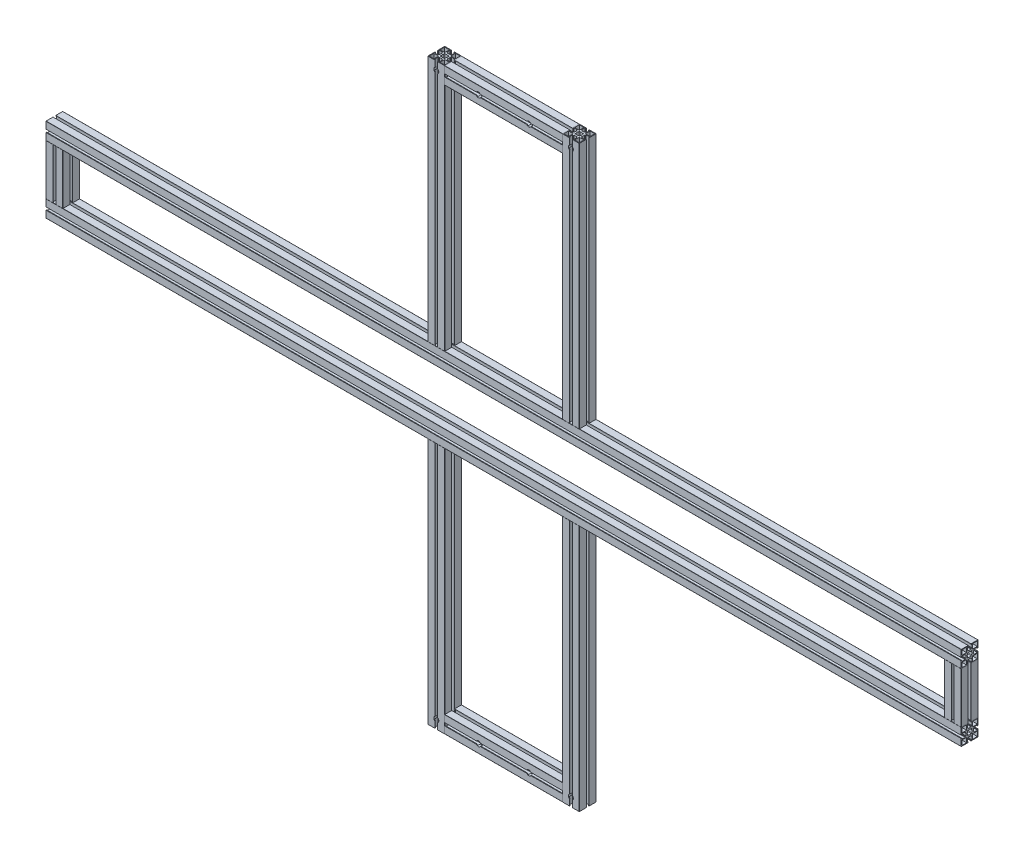
SolidWorks part; units mm, degrees
ref_plane "前视" through (0, 0, 0) normal (0, 0, 1) x (1, 0, 0)
ref_plane "上视" through (0, 0, 0) normal (0, 1, 0) x (1, 0, 0)
ref_plane "右视" through (0, 0, 0) normal (1, 0, 0) x (0, 0, -1)
sketch3d "3D草图1"
  line L0 (0, 0, 0) -> (2670, 0, 0)
  line L1 (2670, 0, 0) -> (2670, -200, 0)
  line L2 (2670, -200, 0) -> (0, -200, 0)
  line L3 (0, -200, 0) -> (0, 0, 0)
  line L4 (1135, 0, 0) -> (1135, 735, 0)
  line L5 (1135, 735, 0) -> (1535, 735, 0)
  line L6 (1535, 735, 0) -> (1535, 0, 0)
  line L7 (1135, -200, 0) -> (1135, -935, 0)
  line L8 (1135, -935, 0) -> (1535, -935, 0)
  line L9 (1535, -935, 0) -> (1535, -200, 0)
  line L10 (1335, 735, 0) -> (1335, 0, 0) construction
  dimension "D1" = 2670
  dimension "D2" = 200
  dimension "D3" = 400
  dimension "D4" = 1670
other "结构构件1"
ref_plane "基准面1" through (2670, -200, 0) normal (-1, 0, 0) x (0, 0, 1)
sketch "Sketch13" plane through (2670, -200, 0) normal (-1, 0, 0) x (0, 0, 1)
  line L0 (0, 0) -> (0, 16.3773) construction
  line L1 (0, 0) -> (-5.6569, 5.6569) construction
  line L2 (-24.5, 25) -> (-4.25, 25)
  line L3 (-25, 24.5) -> (-25, 4.25)
  line L4 (-24.5, -25) -> (-4.25, -25)
  line L5 (25, 24.5) -> (25, 4.25)
  line L6 (-4.879, 6.4347) -> (-4.1104, 5.6661)
  line L7 (-6.4347, 4.879) -> (-5.6661, 4.1104)
  line L8 (6.4347, 4.879) -> (5.6661, 4.1104)
  line L9 (0, 0) -> (20.7093, 0) construction
  line L10 (4.879, 6.4347) -> (4.1104, 5.6661)
  line L11 (4.879, -6.4347) -> (4.1104, -5.6661)
  line L12 (6.4347, -4.879) -> (5.6661, -4.1104)
  line L13 (-6.4347, -4.879) -> (-5.6661, -4.1104)
  line L14 (-4.879, -6.4347) -> (-4.1104, -5.6661)
  line L15 (-4.25, 25) -> (-4.25, 23.2)
  line L16 (-23, 23) -> (-9, 23)
  line L17 (-23, 23) -> (-23, 9)
  line L18 (-23, 9) -> (-9, 9)
  line L19 (-9, 23) -> (-9, 9)
  line L20 (-6.85, 23.2) -> (-4.25, 23.2)
  line L21 (-6.85, 23.2) -> (-6.85, 13.2)
  line L22 (-6.85, 13.2) -> (-4.25, 13.2)
  line L23 (6.85, 23.2) -> (6.85, 13.2)
  line L24 (4.25, 25) -> (4.25, 23.2)
  line L25 (4.25, 25) -> (24.5, 25)
  line L26 (4.25, 23.2) -> (6.85, 23.2)
  line L27 (9, 23) -> (9, 9)
  line L28 (23, 9) -> (9, 9)
  line L29 (23, 23) -> (23, 9)
  line L30 (23, 23) -> (9, 23)
  line L31 (23.2, 6.85) -> (13.2, 6.85)
  line L32 (23.2, 6.85) -> (23.2, 4.25)
  line L33 (25, 4.25) -> (23.2, 4.25)
  line L34 (13.2, 6.85) -> (13.2, 4.25)
  line L35 (23.2, -6.85) -> (13.2, -6.85)
  line L36 (23.2, -4.25) -> (23.2, -6.85)
  line L37 (25, -4.25) -> (23.2, -4.25)
  line L38 (6.85, -23.2) -> (6.85, -13.2)
  line L39 (6.85, -23.2) -> (4.25, -23.2)
  line L40 (4.25, -25) -> (4.25, -23.2)
  line L41 (6.85, -13.2) -> (4.25, -13.2)
  line L42 (-6.85, -23.2) -> (-6.85, -13.2)
  line L43 (-4.25, -23.2) -> (-6.85, -23.2)
  line L44 (-4.25, -25) -> (-4.25, -23.2)
  line L45 (-23.2, -6.85) -> (-13.2, -6.85)
  line L46 (-23.2, -6.85) -> (-23.2, -4.25)
  line L47 (-25, -4.25) -> (-23.2, -4.25)
  line L48 (-13.2, -6.85) -> (-13.2, -4.25)
  line L49 (-23.2, 6.85) -> (-13.2, 6.85)
  line L50 (-23.2, 4.25) -> (-23.2, 6.85)
  line L51 (-25, 4.25) -> (-23.2, 4.25)
  line L52 (4.25, -25) -> (24.5, -25)
  line L53 (-25, -4.25) -> (-25, -24.5)
  line L54 (25, -4.25) -> (25, -24.5)
  line L55 (23, -23) -> (23, -9)
  line L56 (23, -9) -> (9, -9)
  line L57 (9, -23) -> (9, -9)
  line L58 (23, -23) -> (9, -23)
  line L59 (-9, -23) -> (-9, -9)
  line L60 (-23, -9) -> (-9, -9)
  line L61 (-23, -23) -> (-9, -23)
  line L62 (-23, -23) -> (-23, -9)
  line L63 (-4.25, 13.2) -> (-4.25, 11.4)
  line L64 (-4.25, 11.4) -> (4.25, 11.4)
  line L65 (4.25, 11.4) -> (4.25, 13.2)
  line L66 (4.25, 13.2) -> (6.85, 13.2)
  line L67 (13.2, 4.25) -> (11.4, 4.25)
  line L68 (11.4, 4.25) -> (11.4, -4.25)
  line L69 (11.4, -4.25) -> (13.2, -4.25)
  line L70 (4.25, -13.2) -> (4.25, -11.4)
  line L71 (4.25, -11.4) -> (-4.25, -11.4)
  line L72 (-4.25, -11.4) -> (-4.25, -13.2)
  line L73 (-13.2, -4.25) -> (-11.4, -4.25)
  line L74 (-11.4, -4.25) -> (-11.4, 4.25)
  line L75 (-11.4, 4.25) -> (-13.2, 4.25)
  line L76 (-13.2, 4.25) -> (-13.2, 6.85)
  line L77 (-4.25, -13.2) -> (-6.85, -13.2)
  line L78 (13.2, -4.25) -> (13.2, -6.85)
  arc A0 (-4.1104, 5.6661) -> (4.1104, 5.6661) centre (0, 0) cw
  arc A1 (-4.879, 6.4347) -> (-6.4347, 4.879) centre (-5.6569, 5.6569) ccw
  arc A2 (-4.1104, -5.6661) -> (4.1104, -5.6661) centre (0, 0) ccw
  arc A3 (-5.6661, 4.1104) -> (-5.6661, -4.1104) centre (0, 0) ccw
  arc A4 (6.4347, 4.879) -> (4.879, 6.4347) centre (5.6569, 5.6569) ccw
  arc A5 (4.879, -6.4347) -> (6.4347, -4.879) centre (5.6569, -5.6569) ccw
  arc A6 (-6.4347, -4.879) -> (-4.879, -6.4347) centre (-5.6569, -5.6569) ccw
  arc A7 (5.6661, 4.1104) -> (5.6661, -4.1104) centre (0, 0) cw
  arc A8 (-24.5, 25) -> (-25, 24.5) centre (-24.5, 24.5) ccw
  arc A9 (24.5, 25) -> (25, 24.5) centre (24.5, 24.5) cw
  arc A10 (24.5, -25) -> (25, -24.5) centre (24.5, -24.5) ccw
  arc A11 (-25, -24.5) -> (-24.5, -25) centre (-24.5, -24.5) ccw
  point P88 (-25, 25)
  point P91 (25, 25)
  point P92 (-25, -25)
  point P105 (25, -25)
  point P106 (0, 0)
  dimension "D2" = 7
  dimension "D3" = 45
  dimension "D4" = 1.1
  dimension "D5" = 1.8
  dimension "D6" = 8
  dimension "D7" = 2
  dimension "D8" = 13.7
  dimension "D10" = 10
  dimension "D11" = 14
  dimension "D12" = 50
  dimension "D13" = 8.5
  dimension "D14" = 0.5
  dimension "D9" = 2
other "结构构件2"
ref_plane "基准面2" through (1135, 0, 0) normal (0, 1, 0) x (1, 0, 0)
sketch "Sketch14" plane through (1135, 0, 0) normal (0, 1, 0) x (1, 0, 0)
  line L0 (0, 0) -> (0, 16.3773) construction
  line L1 (0, 0) -> (-5.6569, 5.6569) construction
  line L2 (-24.5, 25) -> (-4.25, 25)
  line L3 (-25, 24.5) -> (-25, 4.25)
  line L4 (-24.5, -25) -> (-4.25, -25)
  line L5 (25, 24.5) -> (25, 4.25)
  line L6 (-4.879, 6.4347) -> (-4.1104, 5.6661)
  line L7 (-6.4347, 4.879) -> (-5.6661, 4.1104)
  line L8 (6.4347, 4.879) -> (5.6661, 4.1104)
  line L9 (0, 0) -> (20.7093, 0) construction
  line L10 (4.879, 6.4347) -> (4.1104, 5.6661)
  line L11 (4.879, -6.4347) -> (4.1104, -5.6661)
  line L12 (6.4347, -4.879) -> (5.6661, -4.1104)
  line L13 (-6.4347, -4.879) -> (-5.6661, -4.1104)
  line L14 (-4.879, -6.4347) -> (-4.1104, -5.6661)
  line L15 (-4.25, 25) -> (-4.25, 23.2)
  line L16 (-23, 23) -> (-9, 23)
  line L17 (-23, 23) -> (-23, 9)
  line L18 (-23, 9) -> (-9, 9)
  line L19 (-9, 23) -> (-9, 9)
  line L20 (-6.85, 23.2) -> (-4.25, 23.2)
  line L21 (-6.85, 23.2) -> (-6.85, 13.2)
  line L22 (-6.85, 13.2) -> (-4.25, 13.2)
  line L23 (6.85, 23.2) -> (6.85, 13.2)
  line L24 (4.25, 25) -> (4.25, 23.2)
  line L25 (4.25, 25) -> (24.5, 25)
  line L26 (4.25, 23.2) -> (6.85, 23.2)
  line L27 (9, 23) -> (9, 9)
  line L28 (23, 9) -> (9, 9)
  line L29 (23, 23) -> (23, 9)
  line L30 (23, 23) -> (9, 23)
  line L31 (23.2, 6.85) -> (13.2, 6.85)
  line L32 (23.2, 6.85) -> (23.2, 4.25)
  line L33 (25, 4.25) -> (23.2, 4.25)
  line L34 (13.2, 6.85) -> (13.2, 4.25)
  line L35 (23.2, -6.85) -> (13.2, -6.85)
  line L36 (23.2, -4.25) -> (23.2, -6.85)
  line L37 (25, -4.25) -> (23.2, -4.25)
  line L38 (6.85, -23.2) -> (6.85, -13.2)
  line L39 (6.85, -23.2) -> (4.25, -23.2)
  line L40 (4.25, -25) -> (4.25, -23.2)
  line L41 (6.85, -13.2) -> (4.25, -13.2)
  line L42 (-6.85, -23.2) -> (-6.85, -13.2)
  line L43 (-4.25, -23.2) -> (-6.85, -23.2)
  line L44 (-4.25, -25) -> (-4.25, -23.2)
  line L45 (-23.2, -6.85) -> (-13.2, -6.85)
  line L46 (-23.2, -6.85) -> (-23.2, -4.25)
  line L47 (-25, -4.25) -> (-23.2, -4.25)
  line L48 (-13.2, -6.85) -> (-13.2, -4.25)
  line L49 (-23.2, 6.85) -> (-13.2, 6.85)
  line L50 (-23.2, 4.25) -> (-23.2, 6.85)
  line L51 (-25, 4.25) -> (-23.2, 4.25)
  line L52 (4.25, -25) -> (24.5, -25)
  line L53 (-25, -4.25) -> (-25, -24.5)
  line L54 (25, -4.25) -> (25, -24.5)
  line L55 (23, -23) -> (23, -9)
  line L56 (23, -9) -> (9, -9)
  line L57 (9, -23) -> (9, -9)
  line L58 (23, -23) -> (9, -23)
  line L59 (-9, -23) -> (-9, -9)
  line L60 (-23, -9) -> (-9, -9)
  line L61 (-23, -23) -> (-9, -23)
  line L62 (-23, -23) -> (-23, -9)
  line L63 (-4.25, 13.2) -> (-4.25, 11.4)
  line L64 (-4.25, 11.4) -> (4.25, 11.4)
  line L65 (4.25, 11.4) -> (4.25, 13.2)
  line L66 (4.25, 13.2) -> (6.85, 13.2)
  line L67 (13.2, 4.25) -> (11.4, 4.25)
  line L68 (11.4, 4.25) -> (11.4, -4.25)
  line L69 (11.4, -4.25) -> (13.2, -4.25)
  line L70 (4.25, -13.2) -> (4.25, -11.4)
  line L71 (4.25, -11.4) -> (-4.25, -11.4)
  line L72 (-4.25, -11.4) -> (-4.25, -13.2)
  line L73 (-13.2, -4.25) -> (-11.4, -4.25)
  line L74 (-11.4, -4.25) -> (-11.4, 4.25)
  line L75 (-11.4, 4.25) -> (-13.2, 4.25)
  line L76 (-13.2, 4.25) -> (-13.2, 6.85)
  line L77 (-4.25, -13.2) -> (-6.85, -13.2)
  line L78 (13.2, -4.25) -> (13.2, -6.85)
  arc A0 (-4.1104, 5.6661) -> (4.1104, 5.6661) centre (0, 0) cw
  arc A1 (-4.879, 6.4347) -> (-6.4347, 4.879) centre (-5.6569, 5.6569) ccw
  arc A2 (-4.1104, -5.6661) -> (4.1104, -5.6661) centre (0, 0) ccw
  arc A3 (-5.6661, 4.1104) -> (-5.6661, -4.1104) centre (0, 0) ccw
  arc A4 (6.4347, 4.879) -> (4.879, 6.4347) centre (5.6569, 5.6569) ccw
  arc A5 (4.879, -6.4347) -> (6.4347, -4.879) centre (5.6569, -5.6569) ccw
  arc A6 (-6.4347, -4.879) -> (-4.879, -6.4347) centre (-5.6569, -5.6569) ccw
  arc A7 (5.6661, 4.1104) -> (5.6661, -4.1104) centre (0, 0) cw
  arc A8 (-24.5, 25) -> (-25, 24.5) centre (-24.5, 24.5) ccw
  arc A9 (24.5, 25) -> (25, 24.5) centre (24.5, 24.5) cw
  arc A10 (24.5, -25) -> (25, -24.5) centre (24.5, -24.5) ccw
  arc A11 (-25, -24.5) -> (-24.5, -25) centre (-24.5, -24.5) ccw
  point P88 (-25, 25)
  point P91 (25, 25)
  point P92 (-25, -25)
  point P105 (25, -25)
  point P106 (0, 0)
  dimension "D2" = 7
  dimension "D3" = 45
  dimension "D4" = 1.1
  dimension "D5" = 1.8
  dimension "D6" = 8
  dimension "D7" = 2
  dimension "D8" = 13.7
  dimension "D10" = 10
  dimension "D11" = 14
  dimension "D12" = 50
  dimension "D13" = 8.5
  dimension "D14" = 0.5
  dimension "D9" = 2
other "剪裁/延伸1"
other "剪裁/延伸2"
other "铝型材 50 X 50L X R0.5(1)"
ref_plane "基准面4" through (1135, 735, 0) normal (1, 0, 0) x (0, 0, -1)
sketch "Sketch1" plane through (1135, 735, 0) normal (1, 0, 0) x (0, 0, -1)
  line L0 (0, 0) -> (0, 16.3773) construction
  line L1 (0, 0) -> (-5.6569, 5.6569) construction
  line L2 (-24.5, 25) -> (-4.25, 25)
  line L3 (-25, 24.5) -> (-25, 4.25)
  line L4 (-24.5, -25) -> (-4.25, -25)
  line L5 (25, 24.5) -> (25, 4.25)
  line L6 (-4.879, 6.4347) -> (-4.1104, 5.6661)
  line L7 (-6.4347, 4.879) -> (-5.6661, 4.1104)
  line L8 (6.4347, 4.879) -> (5.6661, 4.1104)
  line L9 (0, 0) -> (20.7093, 0) construction
  line L10 (4.879, 6.4347) -> (4.1104, 5.6661)
  line L11 (4.879, -6.4347) -> (4.1104, -5.6661)
  line L12 (6.4347, -4.879) -> (5.6661, -4.1104)
  line L13 (-6.4347, -4.879) -> (-5.6661, -4.1104)
  line L14 (-4.879, -6.4347) -> (-4.1104, -5.6661)
  line L15 (-4.25, 25) -> (-4.25, 23.2)
  line L16 (-23, 23) -> (-9, 23)
  line L17 (-23, 23) -> (-23, 9)
  line L18 (-23, 9) -> (-9, 9)
  line L19 (-9, 23) -> (-9, 9)
  line L20 (-6.85, 23.2) -> (-4.25, 23.2)
  line L21 (-6.85, 23.2) -> (-6.85, 13.2)
  line L22 (-6.85, 13.2) -> (-4.25, 13.2)
  line L23 (6.85, 23.2) -> (6.85, 13.2)
  line L24 (4.25, 25) -> (4.25, 23.2)
  line L25 (4.25, 25) -> (24.5, 25)
  line L26 (4.25, 23.2) -> (6.85, 23.2)
  line L27 (9, 23) -> (9, 9)
  line L28 (23, 9) -> (9, 9)
  line L29 (23, 23) -> (23, 9)
  line L30 (23, 23) -> (9, 23)
  line L31 (23.2, 6.85) -> (13.2, 6.85)
  line L32 (23.2, 6.85) -> (23.2, 4.25)
  line L33 (25, 4.25) -> (23.2, 4.25)
  line L34 (13.2, 6.85) -> (13.2, 4.25)
  line L35 (23.2, -6.85) -> (13.2, -6.85)
  line L36 (23.2, -4.25) -> (23.2, -6.85)
  line L37 (25, -4.25) -> (23.2, -4.25)
  line L38 (6.85, -23.2) -> (6.85, -13.2)
  line L39 (6.85, -23.2) -> (4.25, -23.2)
  line L40 (4.25, -25) -> (4.25, -23.2)
  line L41 (6.85, -13.2) -> (4.25, -13.2)
  line L42 (-6.85, -23.2) -> (-6.85, -13.2)
  line L43 (-4.25, -23.2) -> (-6.85, -23.2)
  line L44 (-4.25, -25) -> (-4.25, -23.2)
  line L45 (-23.2, -6.85) -> (-13.2, -6.85)
  line L46 (-23.2, -6.85) -> (-23.2, -4.25)
  line L47 (-25, -4.25) -> (-23.2, -4.25)
  line L48 (-13.2, -6.85) -> (-13.2, -4.25)
  line L49 (-23.2, 6.85) -> (-13.2, 6.85)
  line L50 (-23.2, 4.25) -> (-23.2, 6.85)
  line L51 (-25, 4.25) -> (-23.2, 4.25)
  line L52 (4.25, -25) -> (24.5, -25)
  line L53 (-25, -4.25) -> (-25, -24.5)
  line L54 (25, -4.25) -> (25, -24.5)
  line L55 (23, -23) -> (23, -9)
  line L56 (23, -9) -> (9, -9)
  line L57 (9, -23) -> (9, -9)
  line L58 (23, -23) -> (9, -23)
  line L59 (-9, -23) -> (-9, -9)
  line L60 (-23, -9) -> (-9, -9)
  line L61 (-23, -23) -> (-9, -23)
  line L62 (-23, -23) -> (-23, -9)
  line L63 (-4.25, 13.2) -> (-4.25, 11.4)
  line L64 (-4.25, 11.4) -> (4.25, 11.4)
  line L65 (4.25, 11.4) -> (4.25, 13.2)
  line L66 (4.25, 13.2) -> (6.85, 13.2)
  line L67 (13.2, 4.25) -> (11.4, 4.25)
  line L68 (11.4, 4.25) -> (11.4, -4.25)
  line L69 (11.4, -4.25) -> (13.2, -4.25)
  line L70 (4.25, -13.2) -> (4.25, -11.4)
  line L71 (4.25, -11.4) -> (-4.25, -11.4)
  line L72 (-4.25, -11.4) -> (-4.25, -13.2)
  line L73 (-13.2, -4.25) -> (-11.4, -4.25)
  line L74 (-11.4, -4.25) -> (-11.4, 4.25)
  line L75 (-11.4, 4.25) -> (-13.2, 4.25)
  line L76 (-13.2, 4.25) -> (-13.2, 6.85)
  line L77 (-4.25, -13.2) -> (-6.85, -13.2)
  line L78 (13.2, -4.25) -> (13.2, -6.85)
  arc A0 (-4.1104, 5.6661) -> (4.1104, 5.6661) centre (0, 0) cw
  arc A1 (-4.879, 6.4347) -> (-6.4347, 4.879) centre (-5.6569, 5.6569) ccw
  arc A2 (-4.1104, -5.6661) -> (4.1104, -5.6661) centre (0, 0) ccw
  arc A3 (-5.6661, 4.1104) -> (-5.6661, -4.1104) centre (0, 0) ccw
  arc A4 (6.4347, 4.879) -> (4.879, 6.4347) centre (5.6569, 5.6569) ccw
  arc A5 (4.879, -6.4347) -> (6.4347, -4.879) centre (5.6569, -5.6569) ccw
  arc A6 (-6.4347, -4.879) -> (-4.879, -6.4347) centre (-5.6569, -5.6569) ccw
  arc A7 (5.6661, 4.1104) -> (5.6661, -4.1104) centre (0, 0) cw
  arc A8 (-24.5, 25) -> (-25, 24.5) centre (-24.5, 24.5) ccw
  arc A9 (24.5, 25) -> (25, 24.5) centre (24.5, 24.5) cw
  arc A10 (24.5, -25) -> (25, -24.5) centre (24.5, -24.5) ccw
  arc A11 (-25, -24.5) -> (-24.5, -25) centre (-24.5, -24.5) ccw
  point P88 (-25, 25)
  point P91 (25, 25)
  point P92 (-25, -25)
  point P105 (25, -25)
  point P106 (0, 0)
  dimension "D2" = 7
  dimension "D3" = 45
  dimension "D4" = 1.1
  dimension "D5" = 1.8
  dimension "D6" = 8
  dimension "D7" = 2
  dimension "D8" = 13.7
  dimension "D10" = 10
  dimension "D11" = 14
  dimension "D12" = 50
  dimension "D13" = 8.5
  dimension "D14" = 0.5
  dimension "D9" = 2
other "剪裁/延伸3"
other "剪裁/延伸4"
other "剪裁/延伸5"
other "剪裁/延伸6"
hole_wizard "打孔尺寸(%根据)内六角圆柱头螺钉的类型1" positions "草图1" profile "草图2" counterbore size "M8" standard "GB"
sketch "草图1" plane through (0, 0, 25) normal (0, 0, 1) x (1, 0, 0)
  line L0 (1135, 735) -> (1535, 735) construction
  line L1 (1135, -935) -> (1535, -935) construction
  line L2 (1335, -959.5) -> (1335, -831.815) construction
  line L3 (1510, -959.5) -> (1160, -959.5) construction
  point P0 (1135, 735)
  point P3 (1260, 735)
  point P7 (1410, 735)
  point P9 (1535, 735)
  point P12 (1135, -935)
  point P15 (1260, -935)
  point P19 (1410, -935)
  point P21 (1535, -935)
  dimension "D1" = 150
sketch "草图2" plane through (1135, 735, 25) normal (1, 0, 0) x (0, -1, 0)
  line L0 (0, 0) -> (0, 50)
  line L1 (0, 50) -> (4.5, 50)
  line L3 (4.5, 50) -> (4.5, 9)
  line L4 (4.5, 9) -> (7.5, 9)
  line L5 (7.5, 9) -> (7.5, 0)
  line L7 (7.5, 0) -> (0, 0)
  line L11 (0, -6.35) -> (0, 107.95) construction
  dimension "通孔孔直径" = 9
  dimension "通孔孔深度" = 50
  dimension "柱形沉头孔直径" = 15
  dimension "柱形沉头孔深度" = 9
